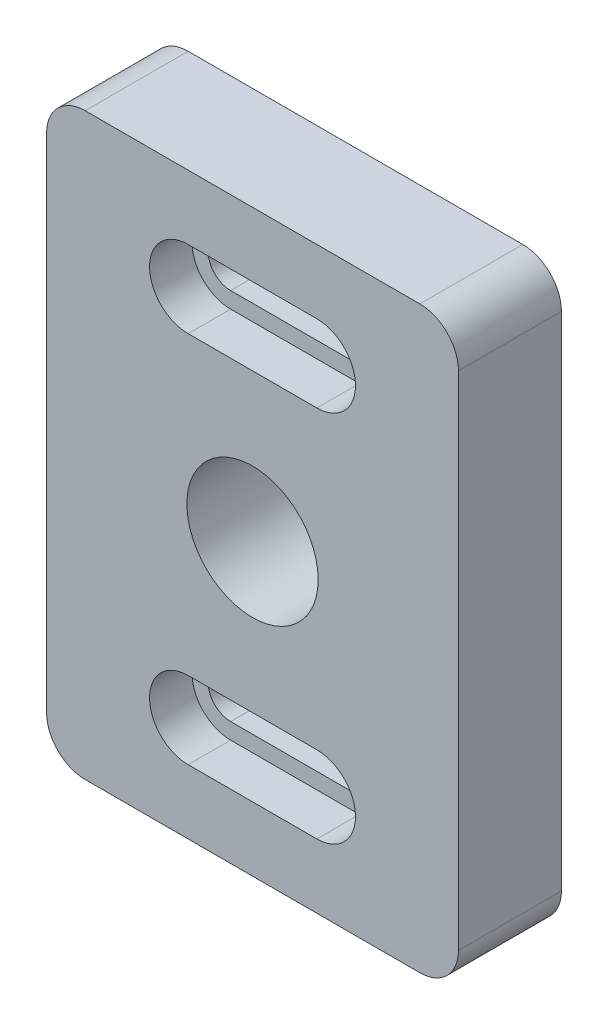
SolidWorks part; units mm, degrees
ref_plane "Front Plane" through (0, 0, 0) normal (0, 0, 1) x (1, 0, 0)
ref_plane "Top Plane" through (0, 0, 0) normal (0, 1, 0) x (1, 0, 0)
ref_plane "Right Plane" through (0, 0, 0) normal (1, 0, 0) x (0, 0, -1)
sketch "Sketch1" plane through (0, 0, 0) normal (0, 0, 1) x (1, 0, 0)
  line L1 (16, -22.5) -> (-16, -22.5)
  line L2 (16, -22.5) -> (16, 22.5)
  line L3 (16, 22.5) -> (-16, 22.5)
  line L4 (-16, -22.5) -> (-16, 22.5)
  line L5 (16, -22.5) -> (-16, 22.5) construction
  line L6 (16, 22.5) -> (-16, -22.5) construction
  point P0 (0, 0)
  dimension "D1" = 32
  dimension "D2" = 45
extrude "Boss-Extrude1" add sketch "Sketch1" along normal blind 8
hole_wizard "M12 Tapped Hole1" positions "Sketch2" profile "Sketch3" tap size "M12" standard "GB" end condition through all
sketch "Sketch2" plane through (0, 0, 8) normal (0, 0, 1) x (1, 0, 0)
  point P0 (0, 0)
sketch "Sketch3" plane through (0, 0, 8) normal (1, 0, 0) x (0, -1, 0)
  line L0 (0, 0) -> (0, 8)
  line L1 (0, 8) -> (5.1, 8)
  line L2 (5.1, 8) -> (5.1, 0)
  line L5 (5.1, 0) -> (0, 0)
  line L11 (0, -6.35) -> (0, 107.95) construction
  dimension "通孔螺纹孔钻头直径" = 10.2
  dimension "通孔螺纹孔钻头深度" = 8
cosmetic thread "Cosmetic Thread1" parameters "D2"=12
sketch "Sketch5" plane through (0, 0, 8) normal (0, 0, 1) x (1, 0, 0)
  line L0 (-5, -14.5) -> (5, -14.5) construction
  line L1 (-5, -12.75) -> (5, -12.75)
  line L2 (-5, -16.25) -> (5, -16.25)
  line L3 (-5, 14.5) -> (5, 14.5) construction
  line L4 (-5, 16.25) -> (5, 16.25)
  line L5 (-5, 12.75) -> (5, 12.75)
  arc A0 (-5, -12.75) -> (-5, -16.25) centre (-5, -14.5) ccw
  arc A1 (5, -16.25) -> (5, -12.75) centre (5, -14.5) ccw
  arc A2 (-5, 16.25) -> (-5, 12.75) centre (-5, 14.5) ccw
  arc A3 (5, 12.75) -> (5, 16.25) centre (5, 14.5) ccw
  point P2 (0, -14.5)
  point P7 (0, 14.5)
  dimension "D5" = 1.75
  dimension "D6" = 1.75
  dimension "D1" = 29
  dimension "D2" = 14.5
  dimension "D3" = 10
  dimension "D4" = 10
extrude "Cut-Extrude1" cut sketch "Sketch5" against normal through all
sketch "Sketch6" plane through (0, 0, 8) normal (0, 0, 1) x (1, 0, 0)
  line L0 (-5, -14.5) -> (5, -14.5) construction
  line L1 (-5, -11.5) -> (5, -11.5)
  line L2 (-5, -17.5) -> (5, -17.5)
  line L3 (-5, 14.5) -> (5, 14.5) construction
  line L4 (-5, 17.5) -> (5, 17.5)
  line L5 (-5, 11.5) -> (5, 11.5)
  arc A0 (-5, -11.5) -> (-5, -17.5) centre (-5, -14.5) ccw
  arc A1 (5, -17.5) -> (5, -11.5) centre (5, -14.5) ccw
  arc A2 (-5, 17.5) -> (-5, 11.5) centre (-5, 14.5) ccw
  arc A3 (5, 11.5) -> (5, 17.5) centre (5, 14.5) ccw
  point P4 (0, -14.5)
  point P9 (0, 14.5)
  dimension "D2" = 3
  dimension "D3" = 3
  dimension "D1" = 10
extrude "Cut-Extrude2" cut sketch "Sketch6" against normal blind 3.3
fillet "Fillet1" radius 3 4 edges at (-16, 22.5, 4) (16, 22.5, 4) (16, -22.5, 4) (-16, -22.5, 4)
